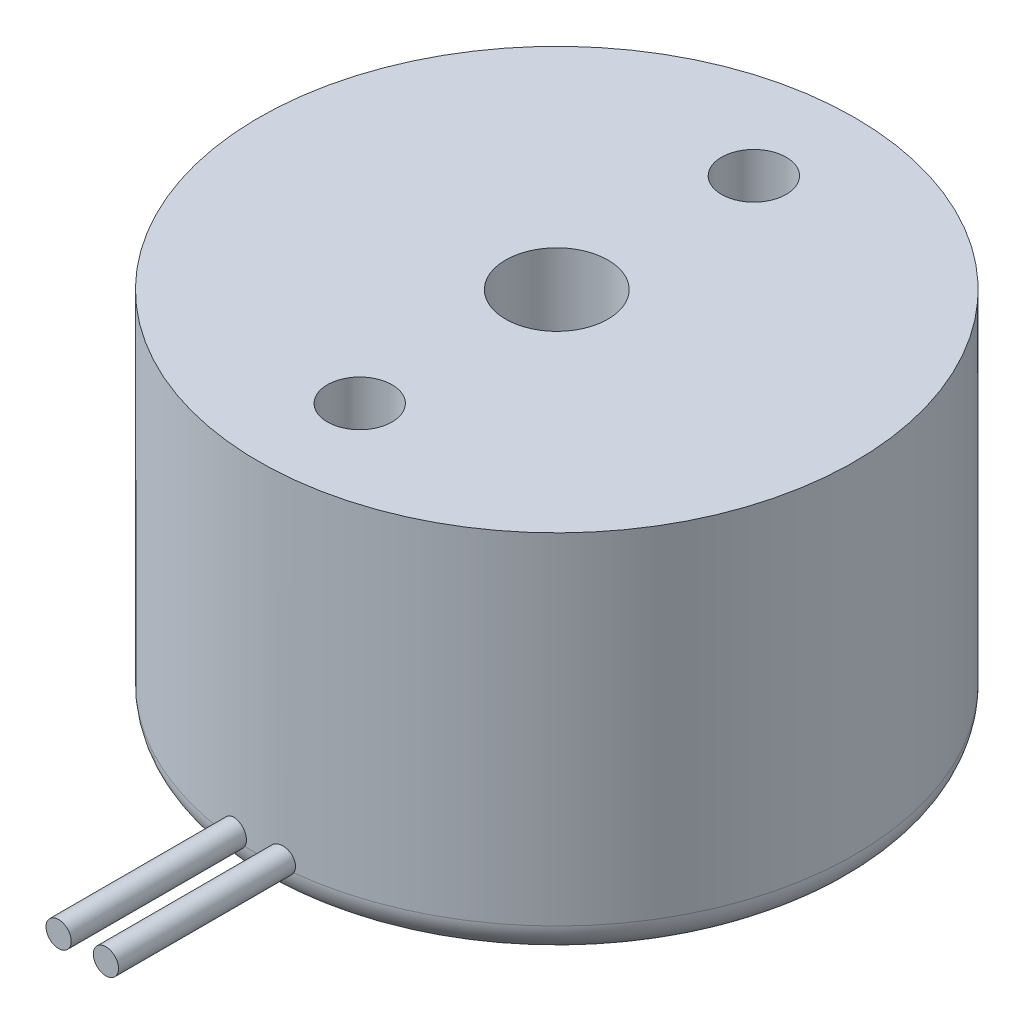
SolidWorks part; units mm, degrees
ref_plane "Front Plane" through (0, 0, 0) normal (0, 0, 1) x (1, 0, 0)
ref_plane "Top Plane" through (0, 0, 0) normal (0, 1, 0) x (1, 0, 0)
ref_plane "Right Plane" through (0, 0, 0) normal (1, 0, 0) x (0, 0, -1)
sketch "Sketch1" plane through (0, 0, 0) normal (0, 0, 1) x (1, 0, 0)
  line L0 (0, 0) -> (0, 19.7567) construction
  line L1 (1.625, 11.8) -> (9.45, 11.8)
  line L2 (9.45, 11.8) -> (9.45, 1)
  line L3 (8.45, 0) -> (4.15, 0)
  line L4 (1.625, 11.8) -> (1.625, 6.3)
  line L5 (4.15, 0) -> (4.15, 6.3)
  line L6 (4.15, 6.3) -> (1.625, 6.3)
  arc A0 (9.45, 1) -> (8.45, 0) centre (8.45, 1) cw
  dimension "D1" = 1
  dimension "D2" = 18.9
  dimension "D3" = 11.8
  dimension "D4" = 3.25
  dimension "D5" = 8.3
  dimension "D6" = 6.3
revolve "Revolve1" add sketch "Sketch1" angle 360 about L0
hole_wizard "M2.5 Tapped Hole1" positions "Sketch3" profile "Sketch2" tap size "M2.5" standard "GB"
sketch "Sketch3" plane through (0, 11.8, 0) normal (0, 1, 0) x (-1, 0, 0)
  line L0 (0, 0) -> (0, -4.1805) construction
  line L2 (0, 0) -> (-2.3138, 0) construction
  point P0 (0, -6.25)
  point P15 (0, 6.25)
  dimension "D1" = 12.5
sketch "Sketch2" plane through (0, 11.8, -6.25) normal (1, 0, 0) x (0, 0, 1)
  line L0 (0, 0) -> (0, 4.9659)
  line L1 (0, 4.9659) -> (1.025, 4.35)
  line L2 (1.025, 4.35) -> (1.025, 0)
  line L5 (1.025, 0) -> (0, 0)
  line L10 (0, 4.9659) -> (-1.025, 4.35) construction
  line L11 (0, -6.35) -> (0, 107.95) construction
  dimension "螺纹孔钻头直径" = 2.05
  dimension "螺纹孔钻头深度" = 4.35
  dimension "导头角度" = 118
cosmetic thread "Cosmetic thread 1" parameters "D1"=3, "D2"=2.5
cosmetic thread "Cosmetic thread 2" parameters "D1"=3, "D2"=2.5
sketch "Sketch5" plane through (0, 0, 0) normal (0, 0, 1) x (1, 0, 0)
  line L0 (-8.45, 0) -> (8.45, 0) construction
  circle A0 centre (-0.8, 1.2) radius 0.4
  circle A1 centre (0.7, 1.2) radius 0.4
  dimension "D1" = 1.5
  dimension "D2" = 0.8
  dimension "D3" = 0.8
  dimension "D4" = 1.2
extrude "Boss-Extrude1" add sketch "Sketch5" along normal blind 15
sketch "Sketch6" plane through (0, 6.3, 0) normal (0, -1, 0) x (1, 0, 0)
  circle A0 centre (0, 0) radius 4.15
extrude "Cut-Extrude2" cut sketch "Sketch6" along normal blind 15
